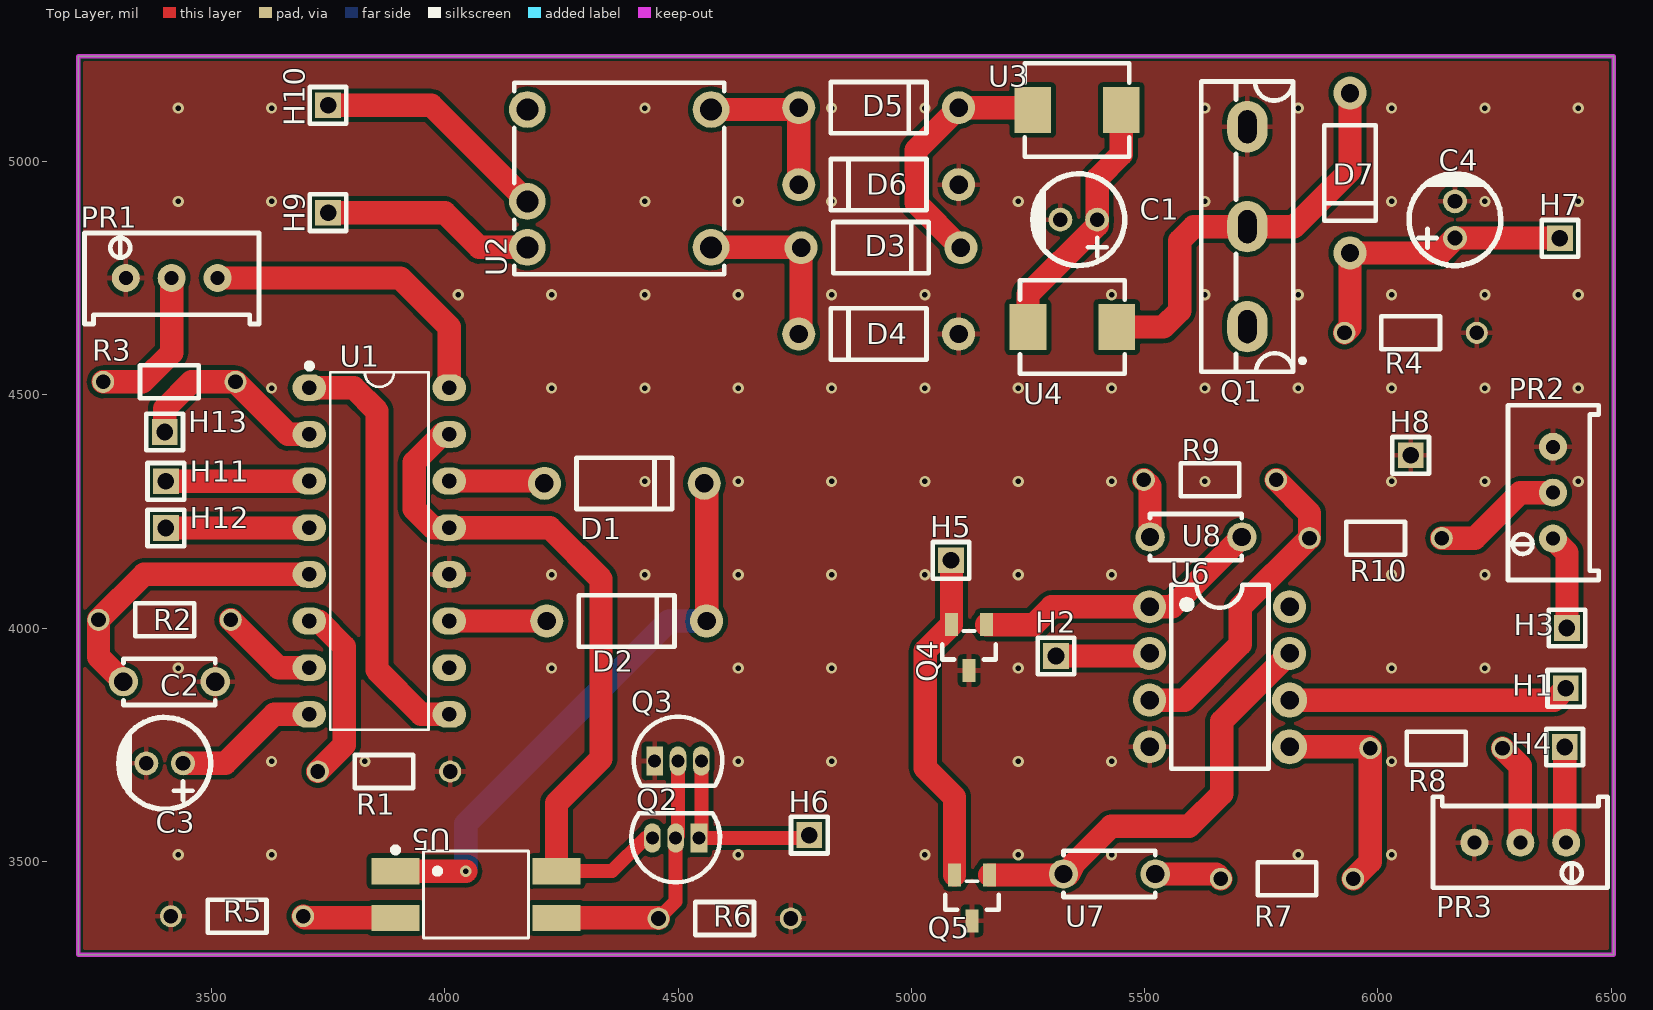
[diagram p0: Top Layer view]
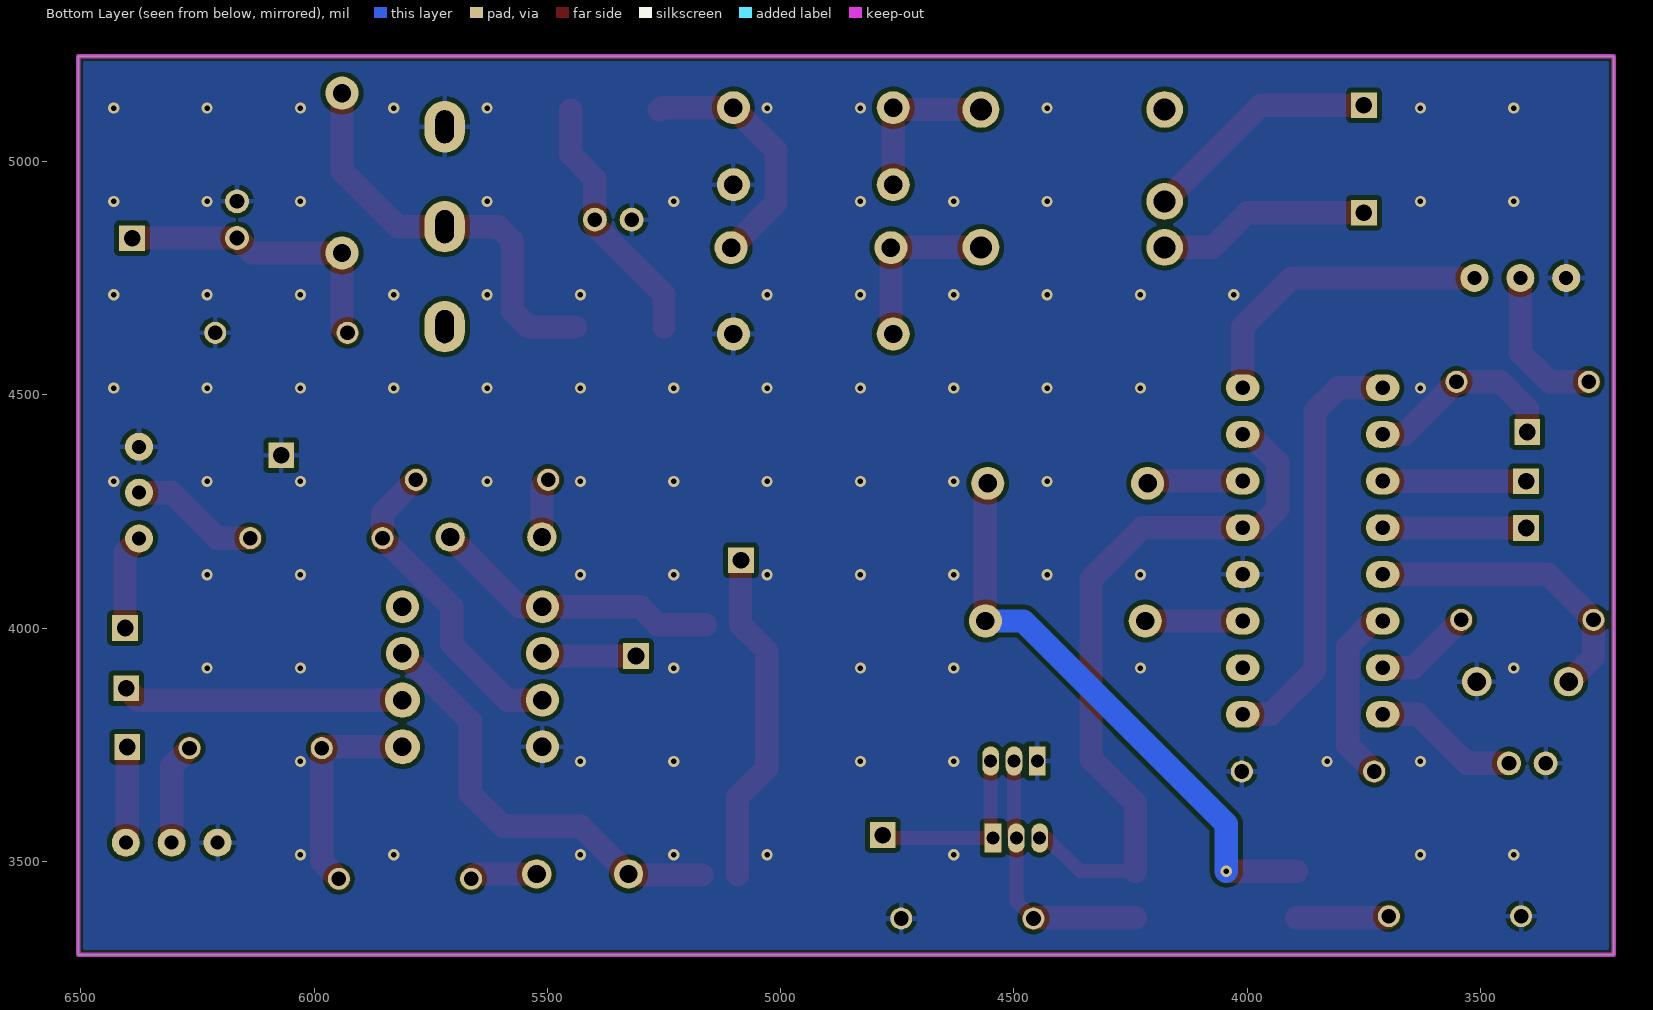
[diagram p1: Bottom Layer view, seen from below]
# Altium PCB MISC51628.pcbdoc
Units mil, origin at the board's own origin, x right, y up, seen from the top; angles counter-clockwise.
Board outline 3290 x 1925 mil, 2 copper layers (Top Layer, Bottom Layer), stack 62.206 mil thick; 50 components, 40 nets, 120 pads, 87 vias.

## Layer stack, top to bottom
Top Solder Mask Layer: solder mask 0.394, Dk 3.3
Top Layer: signal copper 1.379
Dielectric1: surface 59.449, FR4, Dk 4.5
Bottom Layer: signal copper 1.378
Bottom Solder Mask Layer: solder mask 0.394, Dk 3.3

## Board outline
3215,5225 3215,3300 6505,3300 6505,5225

## Design rules (kind name [scope] priority, off if disabled: settings)
BoardOutlineClearance copperThickness2oz_1 [All] p2 off: genericclearance=7.99 ignorepadtopadclearanceinfootprint=FALSE except(0: Arc-SplitContinuation Track-SplitContinuation SMDPad-SplitContinuation THPad-SplitContinuation Via-SplitContinuation Fill-SplitContinuation Region-SplitContinuation Poly-SplitContinuation Text-SplitContinuation Hole-SplitContinuation; 5.98: Arc-CutoutEdge SMDPad-CutoutEdge THPad-CutoutEdge Via-CutoutEdge Fill-CutoutEdge Region-CutoutEdge Text-CutoutEdge; 6.93: Hole-OutlineEdge Hole-CutoutEdge; 10: Poly-OutlineEdge Poly-CutoutEdge; 11.81: Arc-OutlineEdge Track-OutlineEdge SMDPad-OutlineEdge THPad-OutlineEdge Via-OutlineEdge Fill-OutlineEdge Region-OutlineEdge Text-OutlineEdge Track-CutoutEdge)
BoardOutlineClearance copperThickness1oz_1 [All] p4: genericclearance=4.02 ignorepadtopadclearanceinfootprint=FALSE except(0: Arc-SplitContinuation Track-SplitContinuation SMDPad-SplitContinuation THPad-SplitContinuation Via-SplitContinuation Fill-SplitContinuation Region-SplitContinuation Poly-SplitContinuation Text-SplitContinuation Hole-SplitContinuation; 6: SMDPad-CutoutEdge THPad-CutoutEdge Via-CutoutEdge Fill-CutoutEdge Region-CutoutEdge Text-CutoutEdge; 6.93: Hole-OutlineEdge Hole-CutoutEdge; 10: Poly-OutlineEdge Poly-CutoutEdge; 11.8: Arc-OutlineEdge Track-OutlineEdge SMDPad-OutlineEdge THPad-OutlineEdge Via-OutlineEdge Fill-OutlineEdge Region-OutlineEdge Text-OutlineEdge; 11.81: Arc-CutoutEdge Track-CutoutEdge)
Clearance copperThickness2oz [All] p1 off: gap=7.99 ignorepadtopadclearanceinfootprint=FALSE except(5.98: SMDPad-Track SMDPad-SMDPad THPad-Track SMDPad-THPad THPad-THPad Track-Via SMDPad-Via THPad-Via Via-Via Fill-Track Region-Track Fill-SMDPad Region-SMDPad Fill-THPad Region-THPad Fill-Via Region-Via Fill-Fill Fill-Region Region-Region Arc-Track Arc-SMDPad Arc-THPad Arc-Via Fill-Arc Region-Arc Arc-Arc Text-Track SMDPad-Text Text-THPad Text-Via Fill-Text Region-Text Arc-Text Text-Text; 6.93: Hole-Track Hole-SMDPad Hole-THPad Hole-Via Fill-Hole Region-Hole Hole-Arc Hole-Text; 10: Poly-Track Poly-SMDPad Poly-THPad Poly-Via Poly-Fill Poly-Region Poly-Poly Poly-Arc Poly-Text Poly-Hole)
Clearance copperThickness1oz [All] p3: gap=4.02 ignorepadtopadclearanceinfootprint=FALSE except(5.98: SMDPad-Track SMDPad-SMDPad THPad-Track SMDPad-THPad THPad-THPad Track-Via SMDPad-Via THPad-Via Via-Via Fill-Track Region-Track Fill-SMDPad Region-SMDPad Fill-THPad Region-THPad Fill-Via Region-Via Fill-Fill Fill-Region Region-Region; 6: Arc-Track Arc-SMDPad Arc-THPad Arc-Via Fill-Arc Region-Arc Arc-Arc Text-Track SMDPad-Text Text-THPad Text-Via Fill-Text Region-Text Arc-Text Text-Text; 6.93: Hole-Track Hole-SMDPad Hole-THPad Hole-Via Fill-Hole Region-Hole Hole-Arc Hole-Text; 10: Poly-Track Poly-SMDPad Poly-THPad Poly-Via Poly-Fill Poly-Region Poly-Poly Poly-Arc Poly-Text Poly-Hole)
Creepage creepage [All] p1: checkdistance=0 ignoreinternallayers=TRUE applytopolygonpour=TRUE
DiffPairsRouting differentialPair [All] p1: maxlimit=6 minlimit=6 mostfreqgap=6 toplayer_minwidth=5 toplayer_prefwidth=10 toplayer_maxwidth=100 toplayer_mingap=6 toplayer_prefgap=6 toplayer_maxgap=6 bottomlayer_minwidth=5 bottomlayer_prefwidth=10 bottomlayer_maxwidth=100 bottomlayer_mingap=6 bottomlayer_prefgap=6 bottomlayer_maxgap=6 maxuncoupledlength=10
HoleToHoleClearance otherClearance [All] p1: gap=11.81 allowstackedmicrovias=TRUE
Length netLength [All] p1: minlimit=0 maxlimit=0
MatchedLengths netLengthTolerance [All] p1: tolerance=1000
PasteMaskExpansion pasteMaskExpansion [All] p1: expansion=0
PlaneConnect innerPlane [All] p1: planeconnectstyle=Relief reliefexpansion=20 reliefentries=4 reliefconductorwidth=10 reliefairgap=10
PolygonConnect copperRegion [(InNet('GND'))] p1: connectstyle=Relief reliefconductorwidth=10 reliefentries=4 polygonreliefangle="90 Angle" airgapwidth=10 via.connectstyle=Relief via.reliefconductorwidth=10 via.reliefentries=4 via.polygonreliefangle="90 Angle" via.airgapwidth=10
RoutingVias viaSize [All] p1: holewidth=12.01 width=24.02 viastyle="Through Hole" minholewidth=11.81 minwidth=19.68 maxholewidth=248.03 maxwidth=393.7
SolderMaskExpansion solderMaskExpansion [IsVia] p1: expansion=-1000 istentingtop=TRUE
SolderMaskExpansion solderMaskExpansion [All] p2: expansion=2 istentingtop=FALSE
Width copperThickness2oz_2 [All] p1 off: maxlimit=100 minlimit=8 preferedwidth=10
Width copperThickness1oz_2 [All] p2: maxlimit=100 minlimit=5 preferedwidth=10

## Components (designator, comment, footprint, x,y, rotation, side; value= is the part's Value field where it differs from the comment)
C1 "10uF" CAP-TH_BD5.0-P2.00-D0.8-FD-10UF50VC110GL 5358.74,4875 r180 top
C2 "100nF" CAP-TH_L5.0-W2.5-P5.00-D1.0 3410,3885 r0 top
C3 "10uF" CAP-TH_BD5.0-P2.00-D0.8-FD-10UF50VC110GL 3400,3710 r180 top
C4 "10uF" CAP-TH_BD5.0-P2.00-D0.8-FD-10UF50VC110GL 6165,4875 r90 top
D1 "" DO_1N4007 4385,4310 r180 top
D2 "" DO_1N4007 4390,4015 r180 top
D3 "" DO_1N4007 4935,4815 r180 top
D4 "" DO_1N4007 4930,4630 r0 top
D5 "" DO_1N4007 4930,5115 r180 top
D6 "" DO_1N4007 4930,4950 r0 top
D7 "" DO_1N4007 5940,4975 r90 top
H1 "" HDR-TH_1P-V-M_XKB_X4611WV-01I-C28D40 6402.57,3870.8 r0 top
H2 "" HDR-TH_1P-V-M_XKB_X4611WV-01I-C28D40 5310,3940 r0 top
H3 "" HDR-TH_1P-V-M_XKB_X4611WV-01I-C28D40 6405,4000 r0 top
H4 "" HDR-TH_1P-V-M_XKB_X4611WV-01I-C28D40 6400,3745 r0 top
H5 "" HDR-TH_1P-V-M_XKB_X4611WV-01I-C28D40 5085,4145 r0 top
H6 "" HDR-TH_1P-V-M_XKB_X4611WV-01I-C28D40 4781.43,3556.32 r0 top
H7 "" HDR-TH_1P-V-M_XKB_X4611WV-01I-C28D40 6390,4835 r0 top
H8 "" HDR-TH_1P-V-M_XKB_X4611WV-01I-C28D40 6070,4370 r0 top
H9 "" HDR-TH_1P-V-M_XKB_X4611WV-01I-C28D40 3750,4890 r90 top
H10 "" HDR-TH_1P-V-M_XKB_X4611WV-01I-C28D40 3750,5120 r90 top
H11 "" HDR-TH_1P-V-M_XKB_X4611WV-01I-C28D40 3402.68,4314.33 r0 top
H12 "" HDR-TH_1P-V-M_XKB_X4611WV-01I-C28D40 3402.68,4214.33 r0 top
H13 "" HDR-TH_1P-V-M_XKB_X4611WV-01I-C28D40 3400,4420 r0 top
PR1 "10kΩ" R_3296 3415,4755 r0 top
PR2 "10kΩ" R_3296 6370,4290 r90 top
PR3 "10kΩ" R_3296 6305,3535 r180 top
Q1 "IGBT" TO-247-3_L15.9-W5.0-P5.44-L 5720,4860 r90 top
Q2 "" S8050_TO_92 4495,3550 r180 top
Q3 "" S8050_TO_92 4500,3715 r0 top
Q4 "" S8550P_SOT 5123.61,3956.39 r90 top
Q5 "" S8550P_SOT 5130,3420 r90 top
R1 "10kΩ" Res_1/8W 3870,3695 r180 top
R2 "10kΩ" Res_1/8W 3400,4015 r0 top
R3 "10kΩ" Res_1/8W 3410,4525 r0 top
R4 "10kΩ" Res_1/8W 6070,4635 r180 top
R5 "10kΩ" Res_1/8W 3555,3380 r0 top
R6 "10kΩ" Res_1/8W 4600,3380 r180 top
R7 "10kΩ" Res_1/8W 5805,3465 r180 top
R8 "10kΩ" Res_1/8W 6125,3745 r180 top
R9 "10kΩ" Res_1/8W 5640,4320 r180 top
R10 "10kΩ" Res_1/8W 5995,4195 r180 top
U1 "SG3525" DIP-16_L19.2-W6.6-P2.54-LS7.6-BL 3860,4165 r270 top
U2 "LT11-201G" XFMR-TH_LT13-201 4374.05,4963.43 r90 top
U3 "Power inductor (SMD), CKST0502-10uH/M, 10uH, ±20%, 3A, package 5.7mm*5.1mm*2.0mm, Cenke, RoHS" IND-SMD_L5.7-W5.1 5355,5110 r0 top
U4 "Power inductor (SMD), CKST0502-10uH/M, 10uH, ±20%, 3A, package 5.7mm*5.1mm*2.0mm, Cenke, RoHS" IND-SMD_L5.7-W5.1 5345,4645 r0 top
U5 "TLP521" SOP-4_L6.4-W4.6-P2.54-LS10.2-TL 4067.04,3428.86 r0 top
U6 "NE5532AP" PDIP-8_L9.6-W6.4-P2.54-LS7.6-BL 5660.59,3895.54 r270 top
U7 "100nF" CAP-TH_L5.0-W2.5-P5.00-D1.0 5424.42,3472.89 r180 top
U8 "100nF" CAP-TH_L5.0-W2.5-P5.00-D1.0 5610,4195 r0 top

## Footprints (in the part's own frame and the unit in brackets; to place one, negate y for a bottom-side part, rotate by r counter-clockwise, add the part's x,y. Pads: shape width x height; smd on the part's side, far side on the other; paste and mask are expansions set on the pad)
CAP-TH_BD5.0-P2.00-D0.8-FD-10UF50VC110GL [mm]
  round 1.3 hole 0.8: 1(-1,0) 2(1,0)
  silkscreen extent -2.5,-2.5 2.5,2.5
CAP-TH_L5.0-W2.5-P5.00-D1.0 [mm]
  round 1.6 hole 1: 1(-2.5,0) 2(2.5,0)
  silkscreen extent -2.5,-1.27 2.5,1.25
DIP-16_L19.2-W6.6-P2.54-LS7.6-BL [mm]
  oval 1.46x1.825 hole 0.8: 1(-8.89,-3.81) 2(-6.35,-3.81) 3(-3.81,-3.81) 4(-1.27,-3.81) 5(1.27,-3.81) 6(3.81,-3.81) 7(6.35,-3.81) 8(8.89,-3.81) 9(8.89,3.81) 10(6.35,3.81) 11(3.81,3.81) 12(1.27,3.81) 13(-1.27,3.81) 14(-3.81,3.81) 15(-6.35,3.81) 16(-8.89,3.81)
  silkscreen extent -10.22,-3.96 9.73,2.67
DO_1N4007 [mm]
  round 1.8 hole 1 paste+0 mask+0.051: 1(-4.35,0) 2(4.35,0)
  silkscreen extent -2.6,-1.4 2.6,1.4
HDR-TH_1P-V-M_XKB_X4611WV-01I-C28D40 [mm]
  rect 1.4x1.4 hole 0.9: 1(0,0)
  silkscreen extent -1,-1 1,1
IND-SMD_L5.7-W5.1 [mm]
  rect 2x2.5 smd paste+0 mask+0.05: 1(-2.413,0) 2(2.413,0)
  silkscreen extent -2.85,-2.55 2.85,2.55
PDIP-8_L9.6-W6.4-P2.54-LS7.6-BL [mm]
  round 1.8 hole 1: 1(-3.81,-3.81) 2(-1.27,-3.81) 3(1.27,-3.81) 4(3.81,-3.81) 7(-1.27,3.81) 8(-3.81,3.81)
  round 1.905 hole 1: 5(3.81,3.81) 6(1.27,3.81)
  silkscreen extent -5,-2.64 5,2.67
R_3296 [mil]
  round 60 hole 30 paste+0 mask+2: 1(-98.4,-5) 2(0,-5) 3(98.4,-5)
  silkscreen extent -187,-103 187,92
Res_1/8W [mil]
  round 47.2 hole 31.5 paste+0 mask+2: 1(-141.7,2.48) 2(141.7,2.48)
  silkscreen extent -63,-33 63,38
S8050_TO_92 [mil]
  rect 35.4x63 hole 27.6 paste+0 mask+2: 1(-50,0)
  oval 35.4x63 hole 27.6 paste+0 mask+2: 2(0,0) 3(50,0)
  silkscreen extent -95,-53 95,95
S8550P_SOT [mil]
  rect 49.2x27.6 smd paste+0 mask+2: 1(50.84,-37.4) 2(50.84,37.4) 3(-47.56,0)
  silkscreen extent -24,-58 37,58
SOP-4_L6.4-W4.6-P2.54-LS10.2-TL [mil]
  rect 102.36x56 smd: 1(-172.44,50) 2(-172.44,-50) 3(172.44,-50) 4(172.44,50)
  silkscreen extent -178,-93 112,102
TO-247-3_L15.9-W5.0-P5.44-L [mm]
  oval 2.8x2.2 hole 1 slot 1.8 at 0 deg paste+0 mask+0.05: 1(-5.44,0) 2(0,0) 3(5.44,0)
  silkscreen extent -7.9,-3.12 7.9,2.5
XFMR-TH_LT13-201 [mm]
  round 2 hole 1.2: 1(3.75,5) 3(-1.25,5) 4(-3.75,5) 5(-3.75,-5) 8(3.75,-5)
  silkscreen extent -5.21,-5.71 5.21,5.71

## Via types
v1: diameter 24.02, hole 12, Top Layer to Bottom Layer, 87 vias

## Nets (pads, with @x,y where several pads share a name; then routed paths per layer and width w, separated by ;. In a path a pad name is that pad's centre, name@x,y a point inside that pad or via, vN(x,y) a via of type N, cw(c..) or ccw(c..) an arc to the next point about the centre after c; other vN are vias at no path point)
5.1V: PR1.3 U1.16 | length 670.1
  Top Layer w50: PR1.3 3905,4750 4010,4645 U1.16
5V: Q2.3 U1.13 U1.15 U5.4 | length 1562.7
  Top Layer w30: U5.4 4358.86,3478.86 4430,3550 Q2.3
  Top Layer w50: U1.15 3995,4415 3935,4355 3935,4255 3975,4215 U1.13 4225,4215 4335,4105 4335,3720 4239.48,3624.48 U5.4
$1N4: R1.2 U1.6 | length 388.7
  Top Layer w50: U1.6 3730,4015 3785,3960 3785,3749.22 R1.2
$1N5: R2.2 U1.7 | length 210.7
  Top Layer w50: R2.2 3644.18,3915 U1.7
$1N6: C2.1 R2.1 U1.5 | length 646.6
  Top Layer w50: C2.1 3258.3,3938.28 R2.1 3355.82,4115 U1.5
$1N8: U1.1 U1.9 | length 915.1
  Top Layer w50: U1.1 3805,4515 3855,4465 3855,3910 3950,3815 U1.9
$1N10: PR1.2 R3.1 | length 332.6
  Top Layer w50: R3.1 3352.48,4527.48 3415,4590 PR1.2
$1N14: C3.1 U1.8 | length 314.1
  Top Layer w50: C3.1 3530,3710 3635,3815 U1.8
$1N16: D1.2 U1.14 | length 205.8
  Top Layer w50: U1.14 4208.74,4315 D1.2
$1N17: D2.2 U1.11 | length 208.7
  Top Layer w50: U1.11 D2.2
$1N20: D3.2 D4.1 U2.5 | length 380.2
  Top Layer w50: U2.5 4762.95,4815.79 D3.2 4763.74,4635 D4.1
$1N21: D5.2 D6.1 U2.8 | length 354.5
  Top Layer w50: U2.8 4754.8,5111.06 D5.2 D6.1
$1N22: D3.1 D5.1 U3.1 | length 538.5
  Top Layer w50: D3.1 5010,4911.26 5010,5023.74 D5.1 5255,5115 U3.1
$1N23: C1.1 U3.2 U4.1 | length 547.8
  Top Layer w50: U4.1 5250,4715 5398.11,4863.11 C1.1 5398.11,4963.11 5450,5015 U3.2
$1N25: D7.2 Q1.2 U4.2 | length 892.9
  Top Layer w50: U4.2 5540,4645 5575,4680 5575,4830 5605,4860 Q1.2 5820,4860 5940,4980 D7.2
$1N26: C4.1 D7.1 H7.1 R4.2 | length 639.5
  Top Layer w50: R4.2 5940,4644.22 D7.1 6133.11,4803.74 C4.1 6389.37,4835.63 H7.1
$1N28: R5.2 U5.2 | length 199.4
  Top Layer w50: R5.2 3700.32,3378.86 U5.2
$1N29: Q2.2 Q3.2 R6.2 U5.3 | length 574.1
  Top Layer w30: R6.2 4495,3414.22 Q2.2 4500,3555 Q3.2
  Top Layer w50: U5.3 4456.97,3378.86 R6.2
$1N38: Q4.1 U6.1 U8.2 | length 625.2
  Top Layer w50: Q4.1 5262.23,4007.22 5300.54,4045.54 U6.1 5558.96,4045.54 U8.2
$1N39: Q5.1 U6.7 U7.2 | length 935.3
  Top Layer w50: Q5.1 5335.84,3470.84 5349.05,3495.95 5428.11,3575 5595,3575 5665,3645 5665,3799.95 U6.7
$1N40: R7.2 U7.1 | length 144.7
  Top Layer w50: U7.1@5522.85,3472.89 5652.93,3472.89 R7.2
$1N41: R7.1 R8.2 U6.5 | length 469.1
  Top Layer w50: U6.5 5980.29,3745.54 R8.2 5983.3,3499.12 R7.1
$1N42: R9.2 U8.1 | length 128
  Top Layer w50: R9.2 5511.57,4304.25 U8.1
$1N43: R9.1 R10.2 U6.3 | length 688
  Top Layer w50: U6.3 5585.54,3845.54 5705,3965 5705,4045 5852.52,4192.52 R10.2 5853.3,4245.92 R9.1
$1N44: PR2.2 R10.1 | length 278.7
  Top Layer w50: R10.1 6207.52,4192.52 6305,4290 PR2.2
$1N45: PR3.2 R8.1 | length 218.4
  Top Layer w50: R8.1 6305,3704.22 PR3.2
$1N46: H1.1 U6.6 | length 602.5
  Top Layer w50: U6.6 6377.3,3845.54 H1.1
$1N47: H2.1 U6.2 | length 202.9
  Top Layer w50: H2.1 5505.05,3940 U6.2
$1N48: H3.1 PR2.1 | length 204
  Top Layer w50: PR2.1 6405,4161.6 H3.1
$1N49: H4.1 PR3.1 | length 206.4
  Top Layer w50: H4.1 6400,3543.4 PR3.1
$1N52: H9.1 U2.4 | length 457.9
  Top Layer w50: H9.1 4000,4890 4074.21,4815.79 U2.4
$1N53: H10.1 U2.3 | length 512.4
  Top Layer w50: H10.1 3971.42,5120 U2.3
GND: C1.2 C2.2 C3.2 C4.2 D4.2 D6.2 H8.1 PR1.1 PR2.3 PR3.3 Q1.3 Q3.1 Q4.3 Q5.3 R1.1 R4.1 R5.1 R6.1 U1.12 U6.4
  other v1: 3429.1,3514.1 3629.1,3514.1 4629.1,3514.1 5029.1,3514.1 5229.1,3514.1 5429.1,3514.1 5829.1,3514.1 6029.1,3514.1 3629.1,3714.1 3829.1,3714.1 4629.1,3714.1 4829.1,3714.1 5229.1,3714.1 5429.1,3714.1 6029.1,3714.1 3429.1,3914.1 4229.1,3914.1 4629.1,3914.1 4829.1,3914.1 5229.1,3914.1 6029.1,3914.1 6229.1,3914.1 4229.1,4114.1 4429.1,4114.1 4629.1,4114.1 4829.1,4114.1 5029.1,4114.1 5229.1,4114.1 5429.1,4114.1 6029.1,4114.1 6229.1,4114.1 4429.1,4314.1 4629.1,4314.1 4829.1,4314.1 5029.1,4314.1 5229.1,4314.1 5429.1,4314.1 5629.1,4314.1 6029.1,4314.1 6229.1,4314.1 6429.1,4314.1 3629.1,4514.1 4229.1,4514.1 4429.1,4514.1 4629.1,4514.1 4829.1,4514.1 5029.1,4514.1 5229.1,4514.1 5429.1,4514.1 5629.1,4514.1 5829.1,4514.1 6029.1,4514.1 6229.1,4514.1 6429.1,4514.1 4029.1,4714.1 4229.1,4714.1 4429.1,4714.1 4629.1,4714.1 4829.1,4714.1 5029.1,4714.1 5429.1,4714.1 5629.1,4714.1 5829.1,4714.1 6029.1,4714.1 6229.1,4714.1 6429.1,4714.1 3429.1,4914.1 3629.1,4914.1 4429.1,4914.1 4629.1,4914.1 4829.1,4914.1 5229.1,4914.1 5629.1,4914.1 6029.1,4914.1 6229.1,4914.1 6429.1,4914.1 3429.1,5114.1 3629.1,5114.1 4429.1,5114.1 4829.1,5114.1 5029.1,5114.1 5629.1,5114.1 5829.1,5114.1 6029.1,5114.1 6229.1,5114.1 6429.1,5114.1
IN+: H5.1 Q4.2 Q5.2 | length 723.9
  Top Layer w50: H5.1 5086.21,4143.79 Q4.2 5030,3951.01 5030,3700 5092.6,3637.4 Q5.2
N+: H13.1 R3.2 U1.2 | length 430.4
  Top Layer w50: H13.1 3400,4470 3457.48,4527.48 R3.2 3664.18,4415 U1.2
OSCOUT: H12.1 U1.4 | length 307.6
  Top Layer w50: H12.1 3709.33,4214.33 U1.4
PWM: D1.1 D2.1 U5.1 | length 1245.1
  Top Layer w50: U5.1 v1(4045,3478.86) ; D1.1 4561.26,4305 D2.1
  Bottom Layer w50: v1(4045,3478.86) 4045,3580 4480,4015 D2.1
SYNC: H11.1 U1.3 | length 307.6
  Top Layer w50: H11.1 3709.33,4314.33 U1.3
"V G": H6.1 Q2.1 Q3.3 | length 406.1
  Top Layer w30: Q3.3 4550,3555 Q2.1 4775.12,3550 H6.1
VCC: U6.8
pads on no net: Q1.1 U1.10 U2.1

## Polygon pours and split planes (outlines as drawn)
GND on Top Layer (solid, remove dead copper, pour order 0): 3040,5530 3040,3000 6735,3000 6735,5530
GND on Bottom Layer (solid, remove dead copper, pour order 2): 3000,5440 3000,3145 6660,3145 6660,5440

## Keep-outs
Board Outline Layer:
  the board outline again, w10